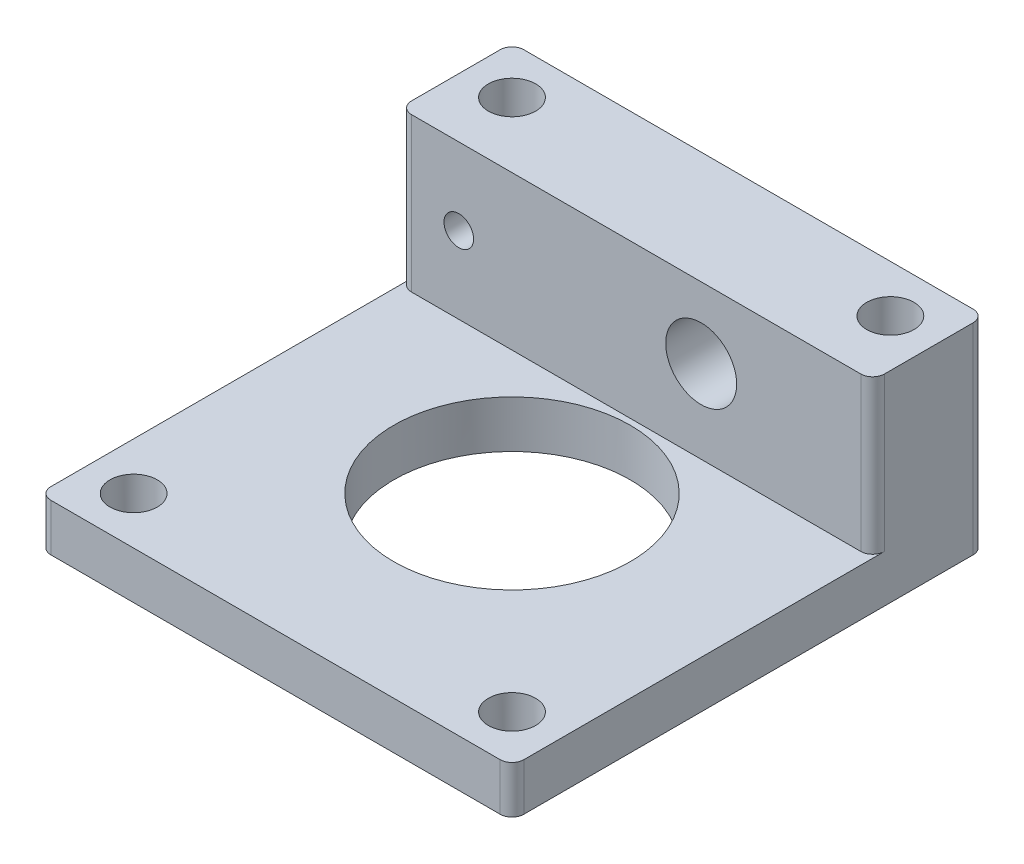
from build123d import *

# Parameters (mm, degrees)
BOSS_EXTRUDE1_DEPTH     = 20
CUT_EXTRUDE1_DEPTH      = 47.572524089
CUT_EXTRUDE1_DEPTH_BACK = 47.572524089
SKETCH2_R               = 10
SKETCH2_R_2             = 2
FILLET1_R               = 1
SKETCH3_R               = 3
SKETCH3_R_2             = 1.25
CUT_EXTRUDE2_DEPTH      = 41.239905566


with BuildPart() as part:
    # Sketch1 → Boss-Extrude1 (new, symmetric)
    with BuildSketch(Plane(origin=(0, 0, 0), x_dir=(0, 0, -1), z_dir=(1, 0, 0))):
        Polygon((0, 0), (40, 0), (40, 4), (40, 17), (30.5, 17), (30.5, 4), (0, 4), align=None)
    extrude(amount=BOSS_EXTRUDE1_DEPTH, both=True)

    # Sketch2 → Cut-Extrude1 (cut, two sides: drawn at the far end of the back side and taken through both)
    with BuildSketch(Plane(origin=(0, 4, 0), x_dir=(1, 0, 0), z_dir=(0, 1, 0)).offset(-CUT_EXTRUDE1_DEPTH_BACK)):
        with Locations(Location((0, 20, 0), (0, 0, 270))):
            Circle(SKETCH2_R)
        with Locations(Location((16, 36, 0), (0, 0, 270))):
            Circle(SKETCH2_R_2)
        with Locations(Location((16, 4, 0), (0, 0, 270))):
            Circle(SKETCH2_R_2)
        with Locations(Location((-16, 4, 0), (0, 0, 270))):
            Circle(SKETCH2_R_2)
        with Locations(Location((-16, 36, 0), (0, 0, 270))):
            Circle(SKETCH2_R_2)
    extrude(amount=CUT_EXTRUDE1_DEPTH + CUT_EXTRUDE1_DEPTH_BACK, mode=Mode.SUBTRACT)

    # Fillet1
    fillet1_edges = [part.edges().sort_by_distance(p)[0] for p in [
        (20, 8.5, -40),
        (20, 10.5, -30.5),
        (20, 2, 0),
        (-20, 10.5, -30.5),
        (-20, 8.5, -40),
        (-20, 2, 0),
    ]]
    fillet(fillet1_edges, radius=FILLET1_R)

    # Sketch3 → Cut-Extrude2 (cut, through all)
    with BuildSketch(Plane.XY.offset(-30.5)):
        with Locations((5.5, 11)):
            Circle(SKETCH3_R)
        with Locations((-15, 10.5)):
            Circle(SKETCH3_R_2)
    extrude(amount=-CUT_EXTRUDE2_DEPTH, mode=Mode.SUBTRACT)


solid = part.part
